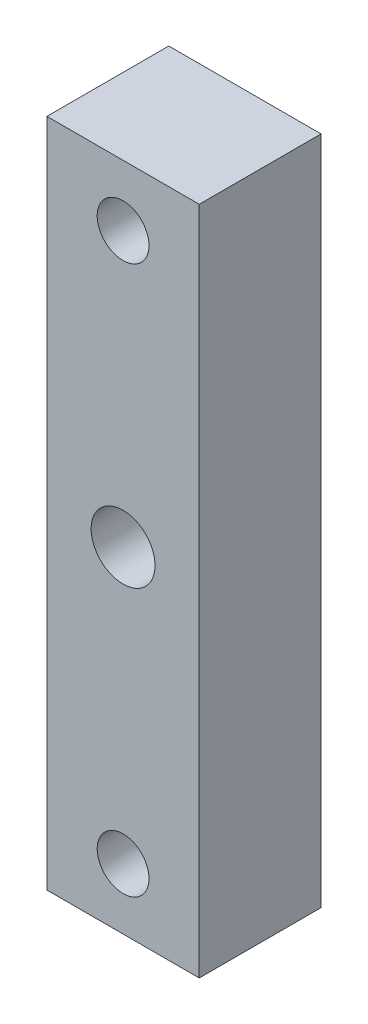
SolidWorks part; units mm, degrees
ref_plane "Front Plane" through (0, 0, 0) normal (0, 0, 1) x (1, 0, 0)
ref_plane "Top Plane" through (0, 0, 0) normal (0, 1, 0) x (1, 0, 0)
ref_plane "Right Plane" through (0, 0, 0) normal (1, 0, 0) x (0, 0, -1)
sketch "Sketch1" plane through (0, 0, 0) normal (0, 0, 1) x (1, 0, 0)
  line L1 (-12.5, -55) -> (12.5, -55)
  line L2 (-12.5, -55) -> (-12.5, 55)
  line L3 (-12.5, 55) -> (12.5, 55)
  line L4 (12.5, -55) -> (12.5, 55)
  line L5 (-12.5, -55) -> (12.5, 55) construction
  line L6 (-12.5, 55) -> (12.5, -55) construction
  point P0 (0, 0)
  dimension "D1" = 25
  dimension "D2" = 110
extrude "Boss-Extrude1" add sketch "Sketch1" along normal blind 20
sketch "Sketch3" plane through (0, 0, 20) normal (0, 0, 1) x (1, 0, 0)
  line L0 (-12.5, 55) -> (-12.5, -55) construction
  line L2 (12.5, 55) -> (-12.5, 55) construction
  line L3 (-12.5, -55) -> (12.5, -55) construction
  circle A3 centre (0, 45) radius 4.25
  circle A4 centre (0, -45) radius 4.25
  dimension "D2" = 10
  dimension "D4" = 8.5
  dimension "D5" = 8.5
  dimension "D15" = 10
  dimension "D9" = 12.5
  dimension "D10" = 12.5
extrude "Cut-Extrude1" cut sketch "Sketch3" against normal blind 30
sketch "Sketch5" plane through (0, 0, 0) normal (0, 0, -1) x (-1, 0, 0)
  circle A3 centre (0, 45) radius 6.5
  circle A4 centre (0, -45) radius 6.5
  dimension "D2" = 13
  dimension "D5" = 13
extrude "Cut-Extrude3" cut sketch "Sketch5" against normal blind 10
hole_wizard "M12x1.25 Tapped Hole1" positions "Sketch7" profile "Sketch6" tap size "M12x1.25" standard "Gb"
sketch "Sketch7" plane through (0, 0, 0) normal (0, 0, -1) x (-1, 0, 0)
  line L0 (12.5, -55) -> (-12.5, -55) construction
  point P6 (0, 0)
  dimension "D1" = 55
sketch "Sketch6" plane through (0, 0, 0) normal (1, 0, 0) x (0, 1, 0)
  line L0 (0, 0) -> (0, 33.4045)
  line L1 (0, 33.4045) -> (5.25, 30.25)
  line L2 (5.25, 30.25) -> (5.25, 0)
  line L5 (5.25, 0) -> (0, 0)
  line L10 (0, 33.4045) -> (-5.25, 30.25) construction
  line L11 (0, -6.35) -> (0, 107.95) construction
  dimension "螺纹孔钻头直径" = 10.5
  dimension "螺纹孔钻头深度" = 30.25
  dimension "导头角度" = 118
cosmetic thread "Cosmetic Thread1" parameters "D1"=20, "D2"=12
